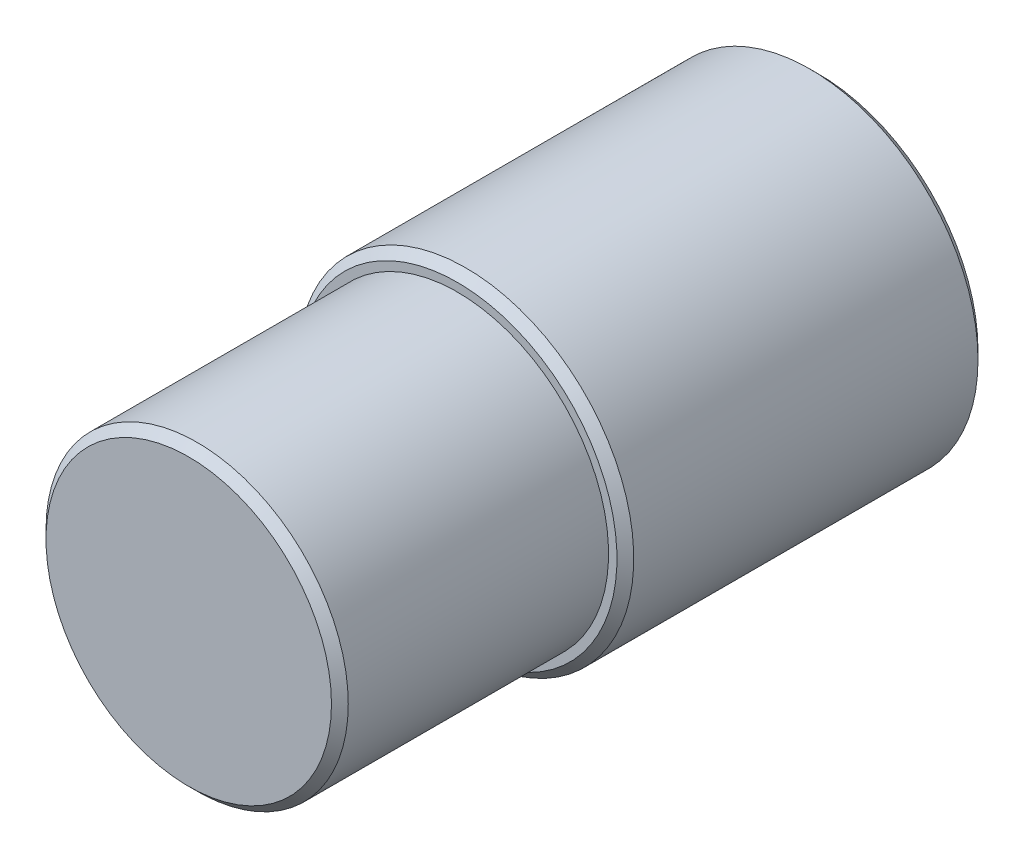
from build123d import *

# Parameters (mm, degrees)
SKETCH1_R           = 9
BOSS_EXTRUDE1_DEPTH = 37.5
SKETCH2_R           = 10
BOSS_EXTRUDE2_DEPTH = 21.5
CHAMFER1_SIZE       = 0.5


with BuildPart() as part:
    # Sketch1 → Boss-Extrude1 (new body)
    with BuildSketch(Plane.XY):
        Circle(SKETCH1_R)
    extrude(amount=BOSS_EXTRUDE1_DEPTH)

    # Sketch2 → Boss-Extrude2 (add)
    with BuildSketch(Plane(origin=(0, 0, 0), x_dir=(-1, 0, 0), z_dir=(0, 0, -1))):
        Circle(SKETCH2_R)
    extrude(amount=-BOSS_EXTRUDE2_DEPTH)

    # Chamfer1
    chamfer1_edges = [part.edges().sort_by_distance(p)[0] for p in [
        (-9, 0, 37.5),
        (10, 0, 21.5),
        (10, 0, 0),
    ]]
    chamfer(chamfer1_edges, length=CHAMFER1_SIZE)


solid = part.part
